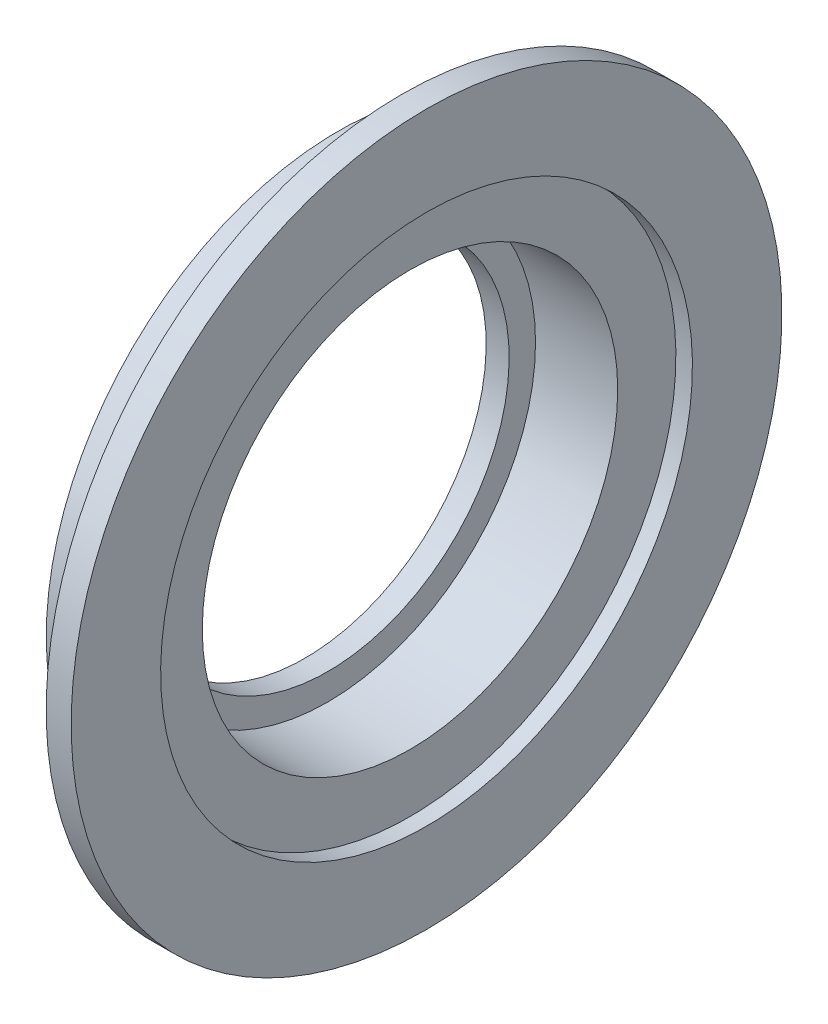
from build123d import *

# Parameters (mm, degrees)
SKETCH2_R           = 34.5
SKETCH2_R_2         = 33.5
SKETCH2_R_3         = 30.5
SKETCH2_R_4         = 29.5
BOSS_EXTRUDE1_DEPTH = 5


with BuildPart() as part:
    # Sketch1 → Revolve1 (revolve)
    with BuildSketch(Plane.XY):
        Polygon((107, 42), (107, 35), (104.508470742, 35), (104.508470742, 27.05), (95.571275451, 27.05), (95.571275451, 21.43258158), (98.286326817, 21.43258158), (98.286326817, 24.55), (108, 24.55), (108, 31.426003585), (109.954236571, 31.426003585), (109.954236571, 42), align=None)
    revolve(axis=Axis((0, 0, 0), (-1, 0, 0)))

    # Sketch2 → Boss-Extrude1 (add)
    # profile 1 of 2: a face of its own
    with BuildSketch(Plane.ZY.offset(-104.508470742)):
        with Locations(Location((0, 0, 0), (0, 0, 270))):
            Circle(SKETCH2_R)
        with Locations(Location((0, 0, 0), (0, 0, 270))):
            Circle(SKETCH2_R_2, mode=Mode.SUBTRACT)
    # profile 2 of 2: a face of its own
    with BuildSketch(Plane.ZY.offset(-104.508470742)):
        with Locations(Location((0, 0, 0), (0, 0, 270))):
            Circle(SKETCH2_R_3)
        with Locations(Location((0, 0, 0), (0, 0, 270))):
            Circle(SKETCH2_R_4, mode=Mode.SUBTRACT)
    extrude(amount=BOSS_EXTRUDE1_DEPTH)


solid = part.part
